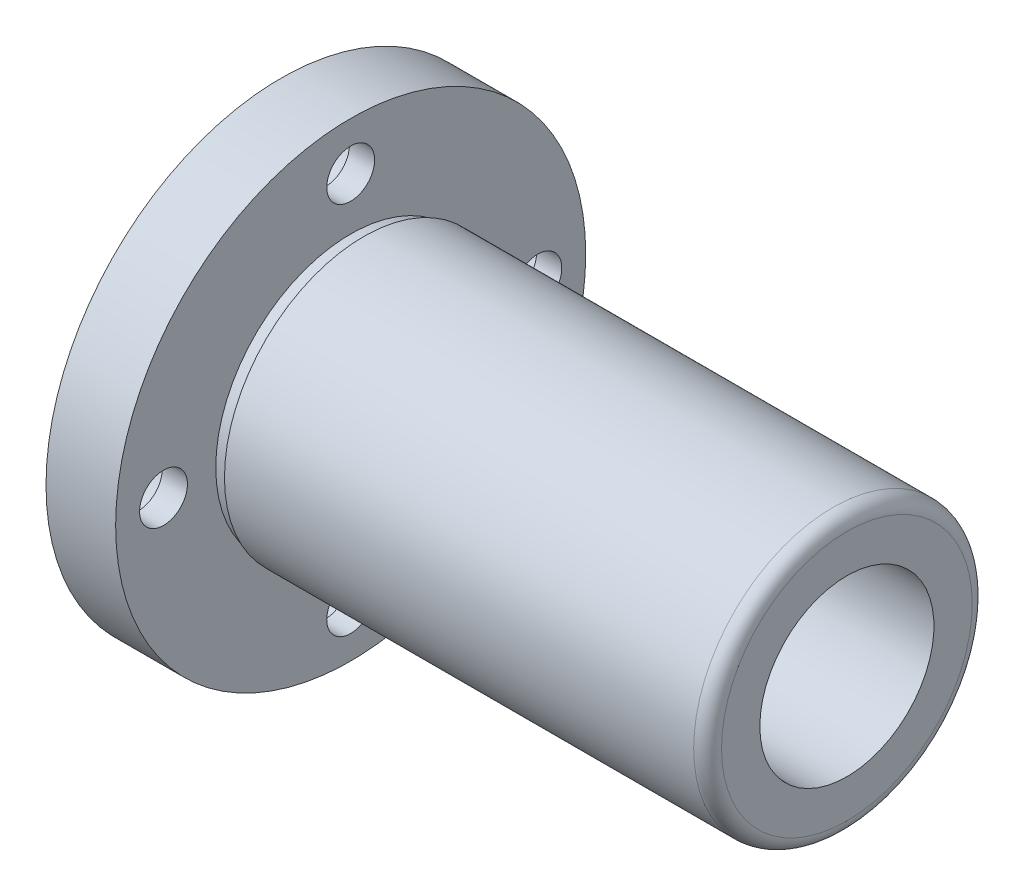
from build123d import *

# Parameters (mm, degrees)
PATTERN_LINEAR_1_COUNT      = 2
PATTERN_LINEAR_1_PITCH      = 30.405591591
PATTERN_LINEAR_1_COUNT_DIR2 = 2
PATTERN_LINEAR_1_PITCH_DIR2 = 30.405591591


with BuildPart() as part:
    # 草图1 → 旋转1 (revolve)
    with BuildSketch(Plane.XY, mode=Mode.PRIVATE) as revolve_1_sk:
        with BuildLine():
            Line((0, 27), (0, 10))
            Line((0, 10), (65, 10))
            Line((65, 10), (65, 14.4))
            ThreePointArc((65, 14.4), (64.53137085, 15.53137085), (63.4, 16))
            Line((63.4, 16), (9.5, 16))
            Line((9.5, 16), (9.5, 15.5))
            Line((9.5, 15.5), (8, 15.5))
            Line((8, 15.5), (8, 27))
            Line((8, 27), (0, 27))
        make_face()
    revolve(revolve_1_sk.sketch.rotate(Axis((65, 0, 0), (-1, 0, 0)), 270), axis=Axis((65, 0, 0), (-1, 0, 0)))

    # 草图2 → 切除-旋转1 (revolve, cut)
    with BuildSketch(Plane.XY, mode=Mode.PRIVATE) as cut_revolve_1_sk:
        Polygon((0, 21.5), (0, 26), (5.1, 26), (5.1, 24.25), (8, 24.25), (8, 21.5), align=None)
    cut_revolve_1 = revolve(cut_revolve_1_sk.sketch.rotate(Axis((8, 21.5, 0), (-1, 0, 0)), 270), axis=Axis((8, 21.5, 0), (-1, 0, 0)), mode=Mode.SUBTRACT)

    # 阵列(线性)1: Cut-Revolve 1 2 × 2
    with Locations(*[Vector(0, -0.7071067811865475, 0.7071067811865477) * (i * PATTERN_LINEAR_1_PITCH) + Vector(0, -0.7071067811865477, -0.7071067811865474) * (j * PATTERN_LINEAR_1_PITCH_DIR2) for i in range(PATTERN_LINEAR_1_COUNT) for j in range(PATTERN_LINEAR_1_COUNT_DIR2) if (i, j) != (0, 0)]):
        add(cut_revolve_1, mode=Mode.SUBTRACT)


solid = part.part
